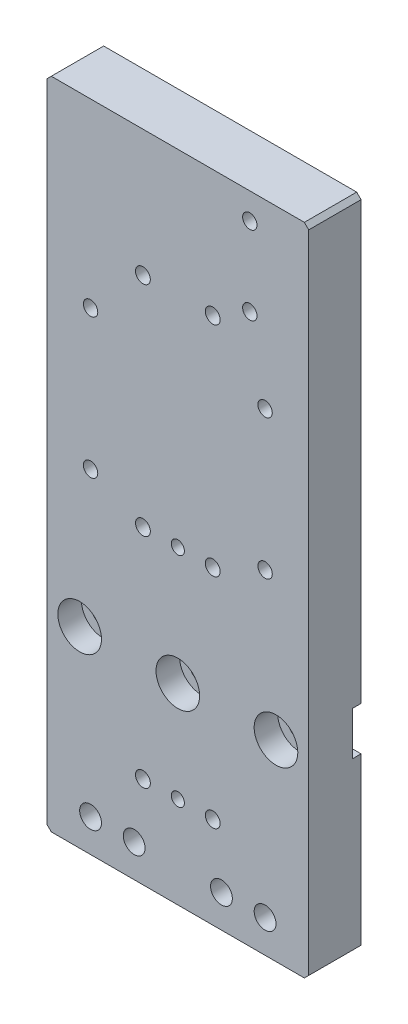
from build123d import *

# Parameters (mm, degrees)
SKETCH1_W                                           = 60
SKETCH1_H                                           = 150
BOSS_EXTRUDE1_DEPTH                                 = 6
M4_TAPPED_HOLE1_D                                   = 3.3
M4_TAPPED_HOLE2_D                                   = 3.3
M4_TAPPED_HOLE2_DEPTH                               = 15.5
M4_TAPPED_HOLE2_TIP                                 = 0.991420021
M6_TAPPED_HOLE2_D                                   = 5
BLIND_PIN_HOLE2_SIZE_MM_D                           = 5
CHAMFER1_SIZE                                       = 1
CBORE_FOR_M3_HEX_SOCKET_HEAD_CAP_SCREW1_D           = 3.4
CBORE_FOR_M3_HEX_SOCKET_HEAD_CAP_SCREW1_CBORE_D     = 6.5
CBORE_FOR_M3_HEX_SOCKET_HEAD_CAP_SCREW1_CBORE_DEPTH = 3.4
LPATTERN1_COUNT                                     = 3
LPATTERN1_PITCH                                     = 50
SKETCH20_R                                          = 1.5
CUT_EXTRUDE1_DEPTH                                  = 82.663945533
SKETCH21_W                                          = 60
SKETCH21_H                                          = 10
CUT_EXTRUDE2_DEPTH                                  = 2
CBORE_FOR_M5_HEX_SOCKET_HEAD_CAP_SCREW1_D           = 5.5
CBORE_FOR_M5_HEX_SOCKET_HEAD_CAP_SCREW1_CBORE_D     = 10
CBORE_FOR_M5_HEX_SOCKET_HEAD_CAP_SCREW1_CBORE_DEPTH = 5.4


with BuildPart() as part:
    # Sketch1 → Boss-Extrude1 (new, symmetric)
    with BuildSketch(Plane.XY):
        Rectangle(SKETCH1_W, SKETCH1_H)
    extrude(amount=BOSS_EXTRUDE1_DEPTH, both=True)

    # M4 Tapped Hole1 (through all)
    with Locations(Plane(origin=(0, 0, -6), x_dir=(-1, 0, 0), z_dir=(0, 0, -1))):
        with Locations((-16.5, 69), (-16.5, 51)):
            Hole(M4_TAPPED_HOLE1_D / 2)

    # M4 Tapped Hole2
    with Locations(Plane(origin=(0, 0, -6), x_dir=(-1, 0, 0), z_dir=(0, 0, -1))):
        with Locations((-20, 33.5), (-20, 1.5), (20, 33.5), (20, 1.5)):
            Hole(M4_TAPPED_HOLE2_D / 2, depth=M4_TAPPED_HOLE2_DEPTH)
            with Locations((0, 0, -(M4_TAPPED_HOLE2_DEPTH + M4_TAPPED_HOLE2_TIP / 2))):  # 118° drill point
                Cone(0, M4_TAPPED_HOLE2_D / 2, M4_TAPPED_HOLE2_TIP, mode=Mode.SUBTRACT)

    # M6 Tapped Hole2 (through all)
    with Locations(Plane(origin=(0, 0, -6), x_dir=(-1, 0, 0), z_dir=(0, 0, -1))):
        with Locations((20, -67.5), (-20, -67.5)):
            Hole(M6_TAPPED_HOLE2_D / 2)

    # Blind Pin Hole2 size mm (through all)
    with Locations(Plane(origin=(0, 0, -6), x_dir=(-1, 0, 0), z_dir=(0, 0, -1))):
        with Locations((10, -67.5), (-10, -67.5)):
            Hole(BLIND_PIN_HOLE2_SIZE_MM_D / 2)

    # Chamfer1
    chamfer1_edges = [part.edges().sort_by_distance(p)[0] for p in [
        (30, -75, 0),
        (-30, -75, 0),
        (-30, 75, 0),
        (30, 75, 0),
    ]]
    chamfer(chamfer1_edges, length=CHAMFER1_SIZE)

    # CBORE for M3 Hex Socket Head Cap Screw1 (through all)
    with Locations(Plane(origin=(0, 0, -6), x_dir=(-1, 0, 0), z_dir=(0, 0, -1))):
        with Locations((8, -54), (-8, -54)):
            cbore_for_m3_hex_socket_head_cap_screw1 = CounterBoreHole(CBORE_FOR_M3_HEX_SOCKET_HEAD_CAP_SCREW1_D / 2, CBORE_FOR_M3_HEX_SOCKET_HEAD_CAP_SCREW1_CBORE_D / 2, CBORE_FOR_M3_HEX_SOCKET_HEAD_CAP_SCREW1_CBORE_DEPTH)

    # LPattern1: CBORE for M3 Hex Socket Head Cap Screw1 ×3
    with Locations(*[(0, i * LPATTERN1_PITCH, 0) for i in range(1, LPATTERN1_COUNT)]):
        add(cbore_for_m3_hex_socket_head_cap_screw1, mode=Mode.SUBTRACT)

    # Sketch20 → Cut-Extrude1 (cut, through all)
    with BuildSketch(Plane(origin=(0, 0, -6), x_dir=(-1, 0, 0), z_dir=(0, 0, -1))):
        with Locations((0, -4)):
            Circle(SKETCH20_R)
        with Locations((0, -54)):
            Circle(SKETCH20_R)
    extrude(amount=-CUT_EXTRUDE1_DEPTH, mode=Mode.SUBTRACT)

    # Sketch21 → Cut-Extrude2 (cut)
    with BuildSketch(Plane(origin=(0, 0, -6), x_dir=(-1, 0, 0), z_dir=(0, 0, -1))):
        with Locations((0, -31)):
            Rectangle(SKETCH21_W, SKETCH21_H)
    extrude(amount=-CUT_EXTRUDE2_DEPTH, mode=Mode.SUBTRACT)

    # CBORE for M5 Hex Socket Head Cap Screw1 (through all)
    with Locations(Plane.XY.offset(6)):
        with Locations((22.5, -31), (0, -31), (-22.5, -31)):
            CounterBoreHole(CBORE_FOR_M5_HEX_SOCKET_HEAD_CAP_SCREW1_D / 2, CBORE_FOR_M5_HEX_SOCKET_HEAD_CAP_SCREW1_CBORE_D / 2, CBORE_FOR_M5_HEX_SOCKET_HEAD_CAP_SCREW1_CBORE_DEPTH)


solid = part.part
